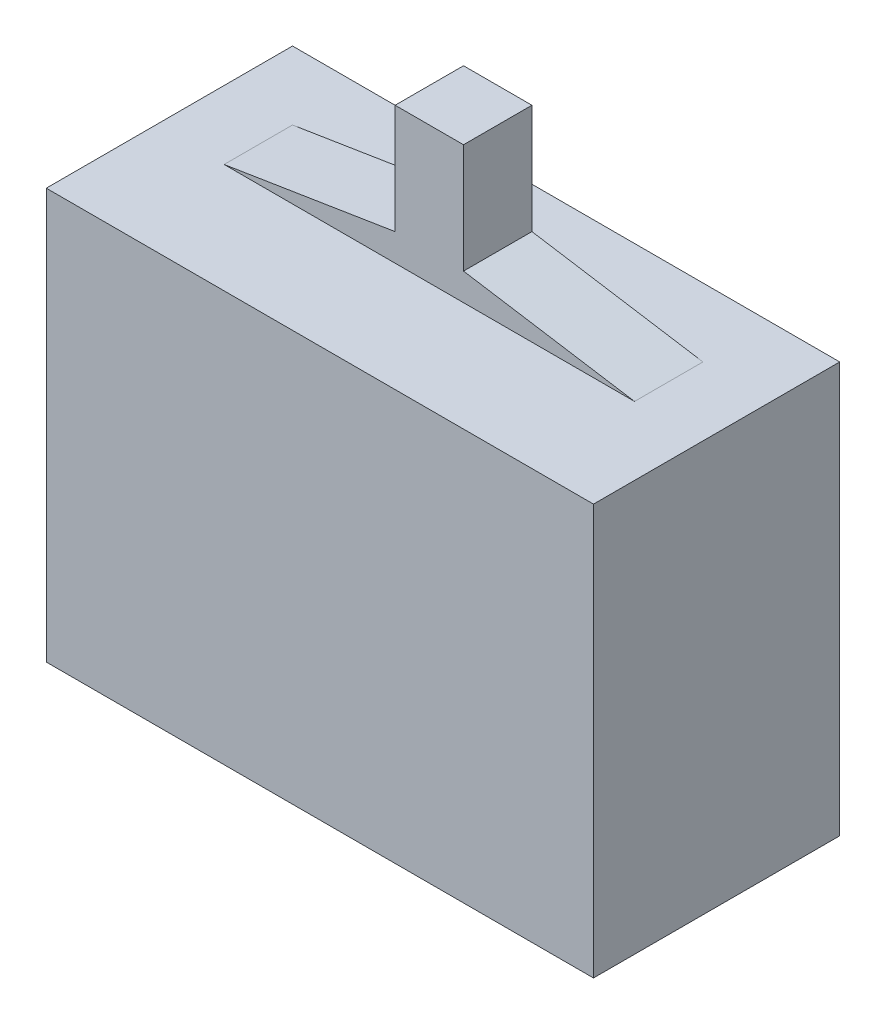
SolidWorks part; units mm, degrees
ref_plane "Front Plane" through (0, 0, 0) normal (0, 0, 1) x (1, 0, 0)
ref_plane "Top Plane" through (0, 0, 0) normal (0, 1, 0) x (1, 0, 0)
ref_plane "Right Plane" through (0, 0, 0) normal (1, 0, 0) x (0, 0, -1)
sketch "Sketch1" plane through (0, 0, 0) normal (0, 0, 1) x (1, 0, 0)
  line L1 (0, 0) -> (40, 0)
  line L2 (0, 0) -> (0, -30)
  line L3 (0, -30) -> (40, -30)
  line L4 (40, 0) -> (40, -30)
  line L5 (0, 0) -> (40, -30) construction
  line L6 (0, -30) -> (40, 0) construction
  point P4 (20, -15)
  dimension "D1" = 30
  dimension "D2" = 40
extrude "Boss-Extrude1" add sketch "Sketch1" along normal blind 18
sketch "Sketch2" plane through (0, 0, 0) normal (0, 0, 1) x (1, 0, 0)
  line L0 (22.5, 2) -> (22.5, 10)
  line L5 (20, 2) -> (20, 0) construction
  line L6 (5, 0) -> (35, 0)
  line L8 (17.5, 2) -> (22.5, 2)
  line L10 (5, 0) -> (22.5, 2) construction
  line L11 (17.5, 2) -> (35, 0) construction
  line L12 (17.5, 2) -> (5, 0)
  line L13 (22.5, 2) -> (35, 0)
  line L14 (22.5, 10) -> (17.5, 10)
  line L15 (17.5, 10) -> (17.5, 2)
  point P4 (20, 1.7143)
  dimension "D2" = 8
  dimension "5" = 5
  dimension "D3" = 2
  dimension "D4" = 30
  dimension "D5" = 5
extrude "Boss-Extrude3" add sketch "Sketch2" along normal blind 5 from offset 5
